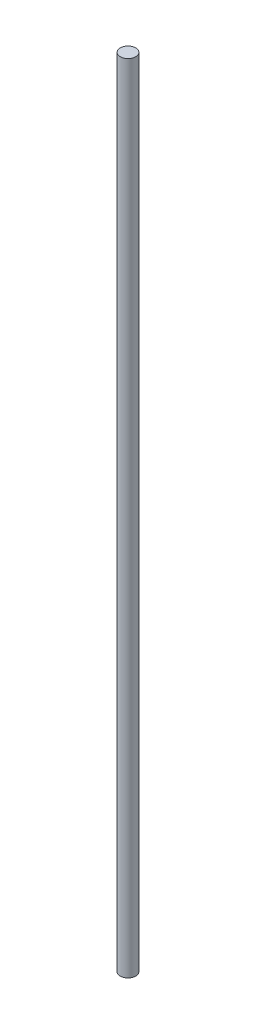
from build123d import *

# Parameters (mm, degrees)
SKETCH_2_R      = 1.5
EXTRUDE_1_DEPTH = 155


with BuildPart() as part:
    # 草图2 → 凸台-拉伸1 (new body)
    with BuildSketch(Plane(origin=(0, 0, 0), x_dir=(1, 0, 0), z_dir=(0, 1, 0))):
        with Locations(Location((0, 0, 0), (0, 0, 270))):
            Circle(SKETCH_2_R)
    extrude(amount=EXTRUDE_1_DEPTH)


solid = part.part
